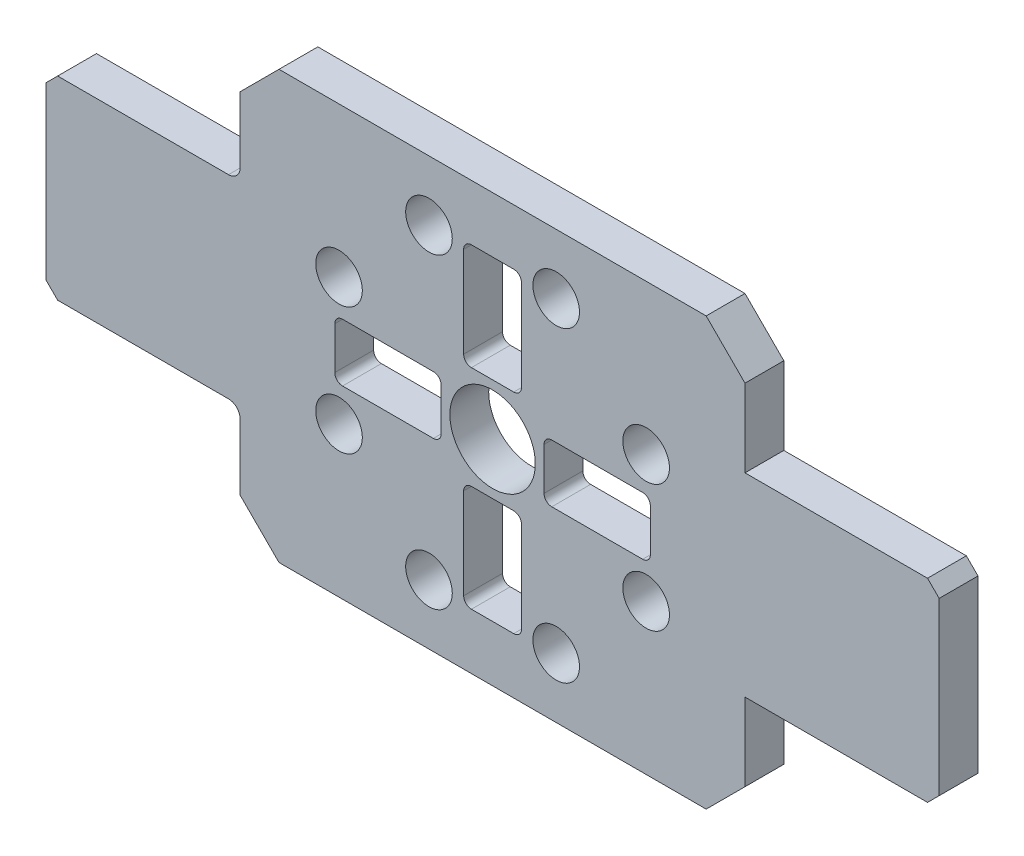
from build123d import *

# Parameters (mm, degrees)
SKETCH1_R               = 6
BOSS_EXTRUDE1_DEPTH     = 10
BOSS_EXTRUDE2_DEPTH     = 10
FILLET1_R               = 3
CUT_EXTRUDE1_DEPTH      = 128.867118525
CUT_EXTRUDE1_DEPTH_BACK = 10
SKETCH3_R               = 11


with BuildPart() as part:
    # Sketch1 → Boss-Extrude1 (new body)
    with BuildSketch(Plane.XY):
        Polygon((-65, 45), (-55, 55), (55, 55), (65, 45), (65, -45), (55, -55), (-55, -55), (-65, -45), align=None)
        with Locations((16.378850905, 39.542043991)):
            Circle(SKETCH1_R, mode=Mode.SUBTRACT)
        with Locations((39.542043991, 16.378850905)):
            Circle(SKETCH1_R, mode=Mode.SUBTRACT)
        with Locations((39.542043991, -16.378850905)):
            Circle(SKETCH1_R, mode=Mode.SUBTRACT)
        with Locations((16.378850905, -39.542043991)):
            Circle(SKETCH1_R, mode=Mode.SUBTRACT)
        with Locations((-16.378850905, -39.542043991)):
            Circle(SKETCH1_R, mode=Mode.SUBTRACT)
        with Locations((-39.542043991, -16.378850905)):
            Circle(SKETCH1_R, mode=Mode.SUBTRACT)
        with Locations((-39.542043991, 16.378850905)):
            Circle(SKETCH1_R, mode=Mode.SUBTRACT)
        with Locations((-16.378850905, 39.542043991)):
            Circle(SKETCH1_R, mode=Mode.SUBTRACT)
        with BuildLine():
            Line((5.447198752, 40.634715337), (-5.447198752, 40.634715337))
            ThreePointArc((-5.447198752, 40.634715337), (-6.861412314, 40.0489289), (-7.447198752, 38.634715337))
            Line((-7.447198752, 38.634715337), (-7.447198752, 15.245017914))
            ThreePointArc((-7.447198752, 15.245017914), (-6.861412314, 13.830804352), (-5.447198752, 13.245017914))
            Line((-5.447198752, 13.245017914), (5.447198752, 13.245017914))
            ThreePointArc((5.447198752, 13.245017914), (6.861412314, 13.830804352), (7.447198752, 15.245017914))
            Line((7.447198752, 15.245017914), (7.447198752, 38.634715337))
            ThreePointArc((7.447198752, 38.634715337), (6.861412314, 40.0489289), (5.447198752, 40.634715337))
        make_face(mode=Mode.SUBTRACT)
        with BuildLine():
            Line((15.245017914, -7.447198752), (38.634715337, -7.447198752))
            ThreePointArc((38.634715337, -7.447198752), (40.0489289, -6.861412314), (40.634715337, -5.447198752))
            Line((40.634715337, -5.447198752), (40.634715337, 5.447198752))
            ThreePointArc((40.634715337, 5.447198752), (40.0489289, 6.861412314), (38.634715337, 7.447198752))
            Line((38.634715337, 7.447198752), (15.245017914, 7.447198752))
            ThreePointArc((15.245017914, 7.447198752), (13.830804352, 6.861412314), (13.245017914, 5.447198752))
            Line((13.245017914, 5.447198752), (13.245017914, -5.447198752))
            ThreePointArc((13.245017914, -5.447198752), (13.830804352, -6.861412314), (15.245017914, -7.447198752))
        make_face(mode=Mode.SUBTRACT)
        with BuildLine():
            Line((-7.447198752, -15.245017914), (-7.447198752, -38.634715337))
            ThreePointArc((-7.447198752, -38.634715337), (-6.861412314, -40.0489289), (-5.447198752, -40.634715337))
            Line((-5.447198752, -40.634715337), (5.447198752, -40.634715337))
            ThreePointArc((5.447198752, -40.634715337), (6.861412314, -40.0489289), (7.447198752, -38.634715337))
            Line((7.447198752, -38.634715337), (7.447198752, -15.245017914))
            ThreePointArc((7.447198752, -15.245017914), (6.861412314, -13.830804352), (5.447198752, -13.245017914))
            Line((5.447198752, -13.245017914), (-5.447198752, -13.245017914))
            ThreePointArc((-5.447198752, -13.245017914), (-6.861412314, -13.830804352), (-7.447198752, -15.245017914))
        make_face(mode=Mode.SUBTRACT)
        with BuildLine():
            Line((-15.245017914, 7.447198752), (-38.634715337, 7.447198752))
            ThreePointArc((-38.634715337, 7.447198752), (-40.0489289, 6.861412314), (-40.634715337, 5.447198752))
            Line((-40.634715337, 5.447198752), (-40.634715337, -5.447198752))
            ThreePointArc((-40.634715337, -5.447198752), (-40.0489289, -6.861412314), (-38.634715337, -7.447198752))
            Line((-38.634715337, -7.447198752), (-15.245017914, -7.447198752))
            ThreePointArc((-15.245017914, -7.447198752), (-13.830804352, -6.861412314), (-13.245017914, -5.447198752))
            Line((-13.245017914, -5.447198752), (-13.245017914, 5.447198752))
            ThreePointArc((-13.245017914, 5.447198752), (-13.830804352, 6.861412314), (-15.245017914, 7.447198752))
        make_face(mode=Mode.SUBTRACT)
    extrude(amount=BOSS_EXTRUDE1_DEPTH)

    # Sketch2 → Boss-Extrude2 (add)
    with BuildSketch(Plane.XY):
        Polygon((-112, 25), (-65, 25), (-65, -25), (-112, -25), (-115, -22), (-115, 22), align=None)
        Polygon((115, -22), (112, -25), (65, -25), (65, 25), (112, 25), (115, 22), align=None)
    extrude(amount=BOSS_EXTRUDE2_DEPTH)

    # Fillet1
    fillet1_edges = [part.edges().sort_by_distance(p)[0] for p in [
        (-65, 25, 5),
        (-65, -25, 5),
    ]]
    fillet(fillet1_edges, radius=FILLET1_R)

    # Sketch3 → Cut-Extrude1 (cut, two sides: drawn at the far end of the back side and taken through both)
    with BuildSketch(Plane.XY.offset(10).offset(-CUT_EXTRUDE1_DEPTH_BACK)):
        with Locations(Location((0, 0, 0), (0, 0, 180))):
            Circle(SKETCH3_R)
    extrude(amount=CUT_EXTRUDE1_DEPTH + CUT_EXTRUDE1_DEPTH_BACK, mode=Mode.SUBTRACT)


solid = part.part
